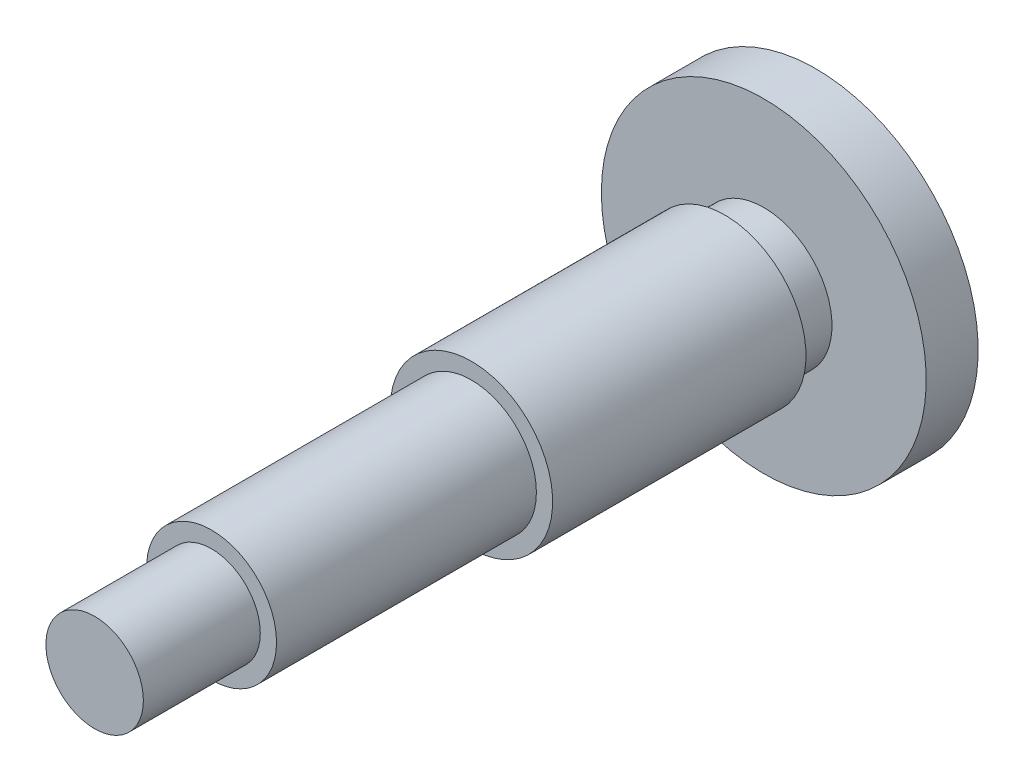
from build123d import *

# Parameters (mm, degrees)
SKETCH_1_R      = 12.5
EXTRUDE_1_DEPTH = 45
SKETCH_2_R      = 25
EXTRUDE_2_DEPTH = 8
SKETCH_3_R      = 10
EXTRUDE_3_DEPTH = 40
SKETCH_5_W      = 2
SKETCH_5_H      = 6
SKETCH_6_R      = 7.5
EXTRUDE_4_DEPTH = 18


with BuildPart() as part:
    # 草图1 → 凸台-拉伸1 (new body)
    with BuildSketch(Plane.XY):
        with Locations(Location((0, 0, 0), (0, 0, 180))):
            Circle(SKETCH_1_R)
    extrude(amount=EXTRUDE_1_DEPTH)

    # 草图2 → 凸台-拉伸2 (add)
    with BuildSketch(Plane(origin=(0, 0, 0), x_dir=(-1, 0, 0), z_dir=(0, 0, -1))):
        Circle(SKETCH_2_R)
    extrude(amount=EXTRUDE_2_DEPTH)

    # 草图3 → 凸台-拉伸3 (add)
    with BuildSketch(Plane.XY.offset(45)):
        Circle(SKETCH_3_R)
    extrude(amount=EXTRUDE_3_DEPTH)

    # 草图5 → 切除-旋转1 (revolve, cut)
    with BuildSketch(Plane(origin=(0, 0, 0), x_dir=(1, 0, 0), z_dir=(0, 1, 0)), mode=Mode.PRIVATE) as cut_revolve_1_sk:
        with Locations((11.5, -3)):
            Rectangle(SKETCH_5_W, SKETCH_5_H)
    revolve(cut_revolve_1_sk.sketch.rotate(Axis((0, 0, 0), (0, 0, 1)), 180), axis=Axis((0, 0, 0), (0, 0, 1)), mode=Mode.SUBTRACT)

    # 草图6 → 凸台-拉伸4 (add)
    with BuildSketch(Plane.XY.offset(85)):
        Circle(SKETCH_6_R)
    extrude(amount=EXTRUDE_4_DEPTH)


solid = part.part
